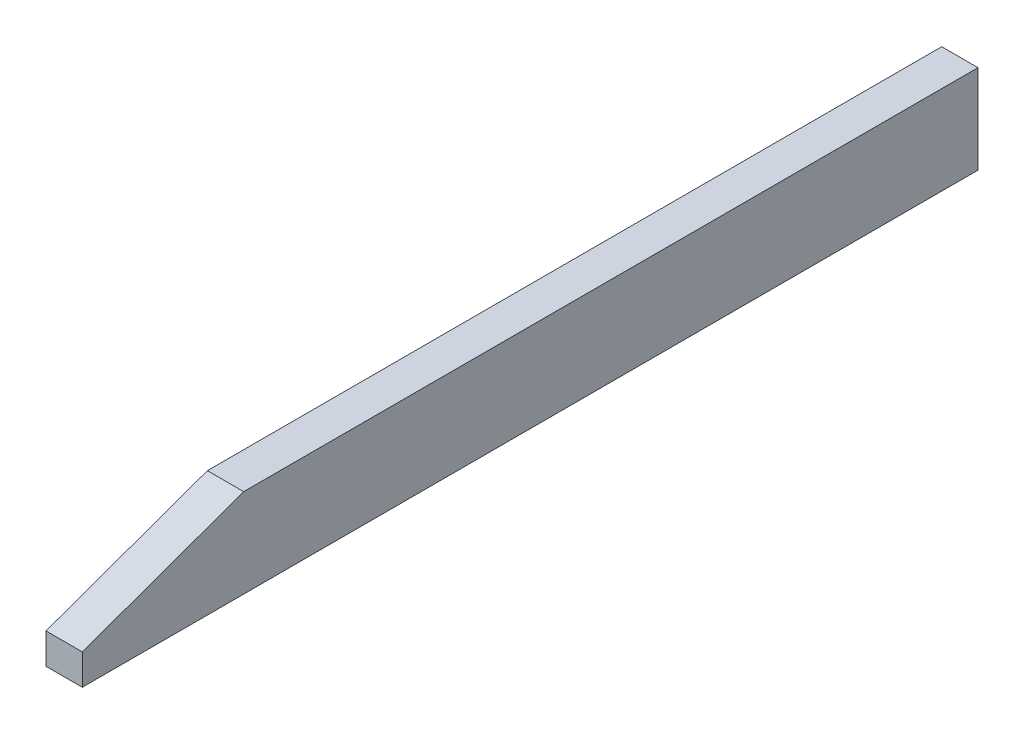
from build123d import *

# Parameters (mm, degrees)
BOSS_EXTRUDE1_DEPTH = 22.5


with BuildPart() as part:
    # Sketch1 → Boss-Extrude1 (new, symmetric)
    with BuildSketch(Plane(origin=(0, 0, 0), x_dir=(0, 0, -1), z_dir=(1, 0, 0))):
        Polygon((0, 0), (1110, 0), (1110, 110), (200, 110), (0, 38), align=None)
    extrude(amount=BOSS_EXTRUDE1_DEPTH, both=True)


solid = part.part
